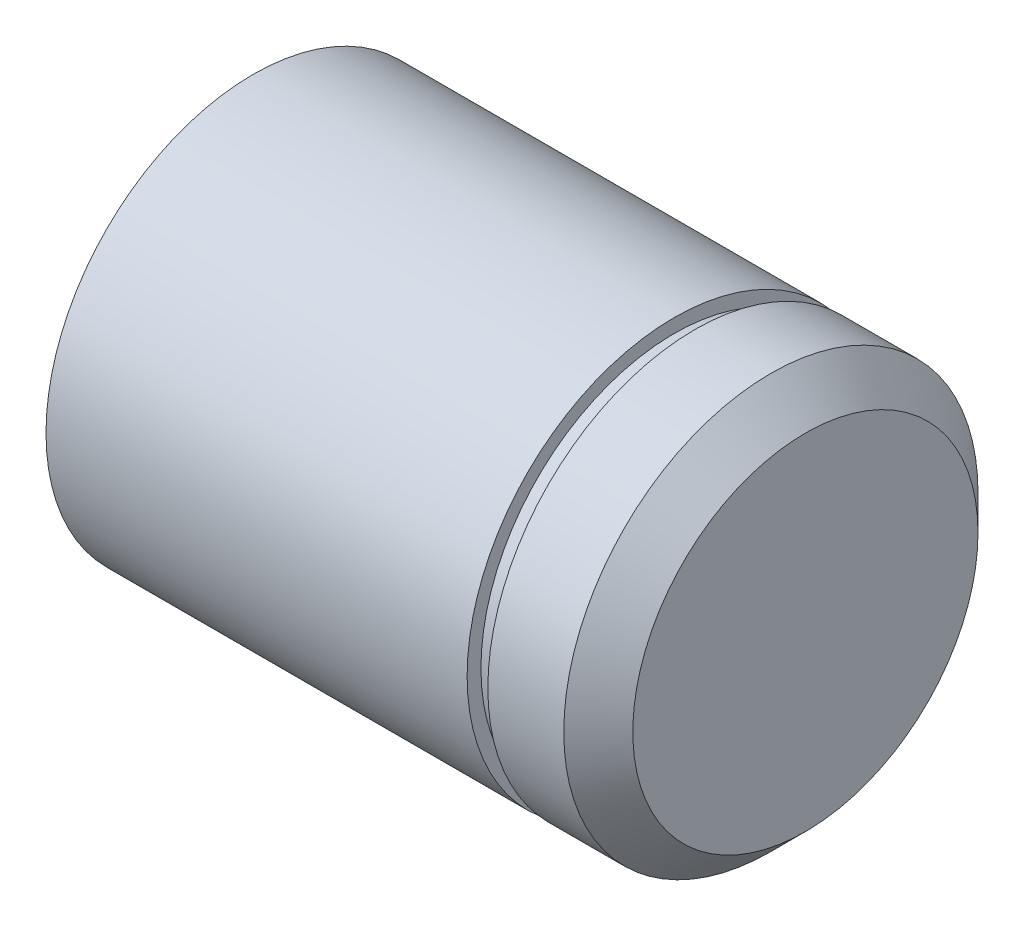
SolidWorks part; units mm, degrees
ref_plane "Front Plane" through (0, 0, 0) normal (0, 0, 1) x (1, 0, 0)
ref_plane "Top Plane" through (0, 0, 0) normal (0, 1, 0) x (1, 0, 0)
ref_plane "Right Plane" through (0, 0, 0) normal (1, 0, 0) x (0, 0, -1)
sketch "Sketch1" plane through (0, 0, 0) normal (1, 0, 0) x (0, 0, -1)
  circle A0 centre (0, 0) radius 3
  dimension "D1" = 6
extrude "Boss-Extrude1" add sketch "Sketch1" along normal blind 8
chamfer "Chamfer1" distance 0.5 angle 45 1 edges at (8, 0, -3)
hole_wizard "M3 Tapped Hole1" positions "3DSketch1" profile "Sketch2" tap size "M3" standard "Gb"
sketch3d "3DSketch1"
  line L0 (7.5, 0, 0) -> (0, 0, 0) construction
  point P0 (0, 0, 0)
  dimension "D1" = 0
sketch "Sketch2" plane through (0, 0, 0) normal (0, 1, 0) x (0, 0, 1)
  line L0 (0, 0) -> (0, 7.2511)
  line L1 (0, 7.2511) -> (1.25, 6.5)
  line L2 (1.25, 6.5) -> (1.25, 0)
  line L5 (1.25, 0) -> (0, 0)
  line L10 (0, 7.2511) -> (-1.25, 6.5) construction
  line L11 (0, -6.35) -> (0, 107.95) construction
  dimension "螺纹孔钻头直径" = 2.5
  dimension "螺纹孔钻头深度" = 6.5
  dimension "导头角度" = 118
cosmetic thread "Hole Thread 1" parameters "D1"=6, "D2"=3
sketch "Sketch3" plane through (0, 0, 0) normal (0, 1, 0) x (1, 0, 0)
  line L0 (0, 0) -> (50000, 0) construction
  line L1 (7.5, 3) -> (0, 3) construction
  line L2 (6.1, 3) -> (6.4, 3)
  line L3 (6.1, 3) -> (6.1, 2.8)
  line L4 (6.1, 2.8) -> (6.4, 2.8)
  line L5 (6.4, 3) -> (6.4, 2.8)
  line L6 (0, 3) -> (0, -3) construction
  dimension "D1" = 6.1
  dimension "D2" = 0.2
  dimension "D3" = 0.3
revolve "Cut-Revolve1" cut sketch "Sketch3" angle 360 about L0
